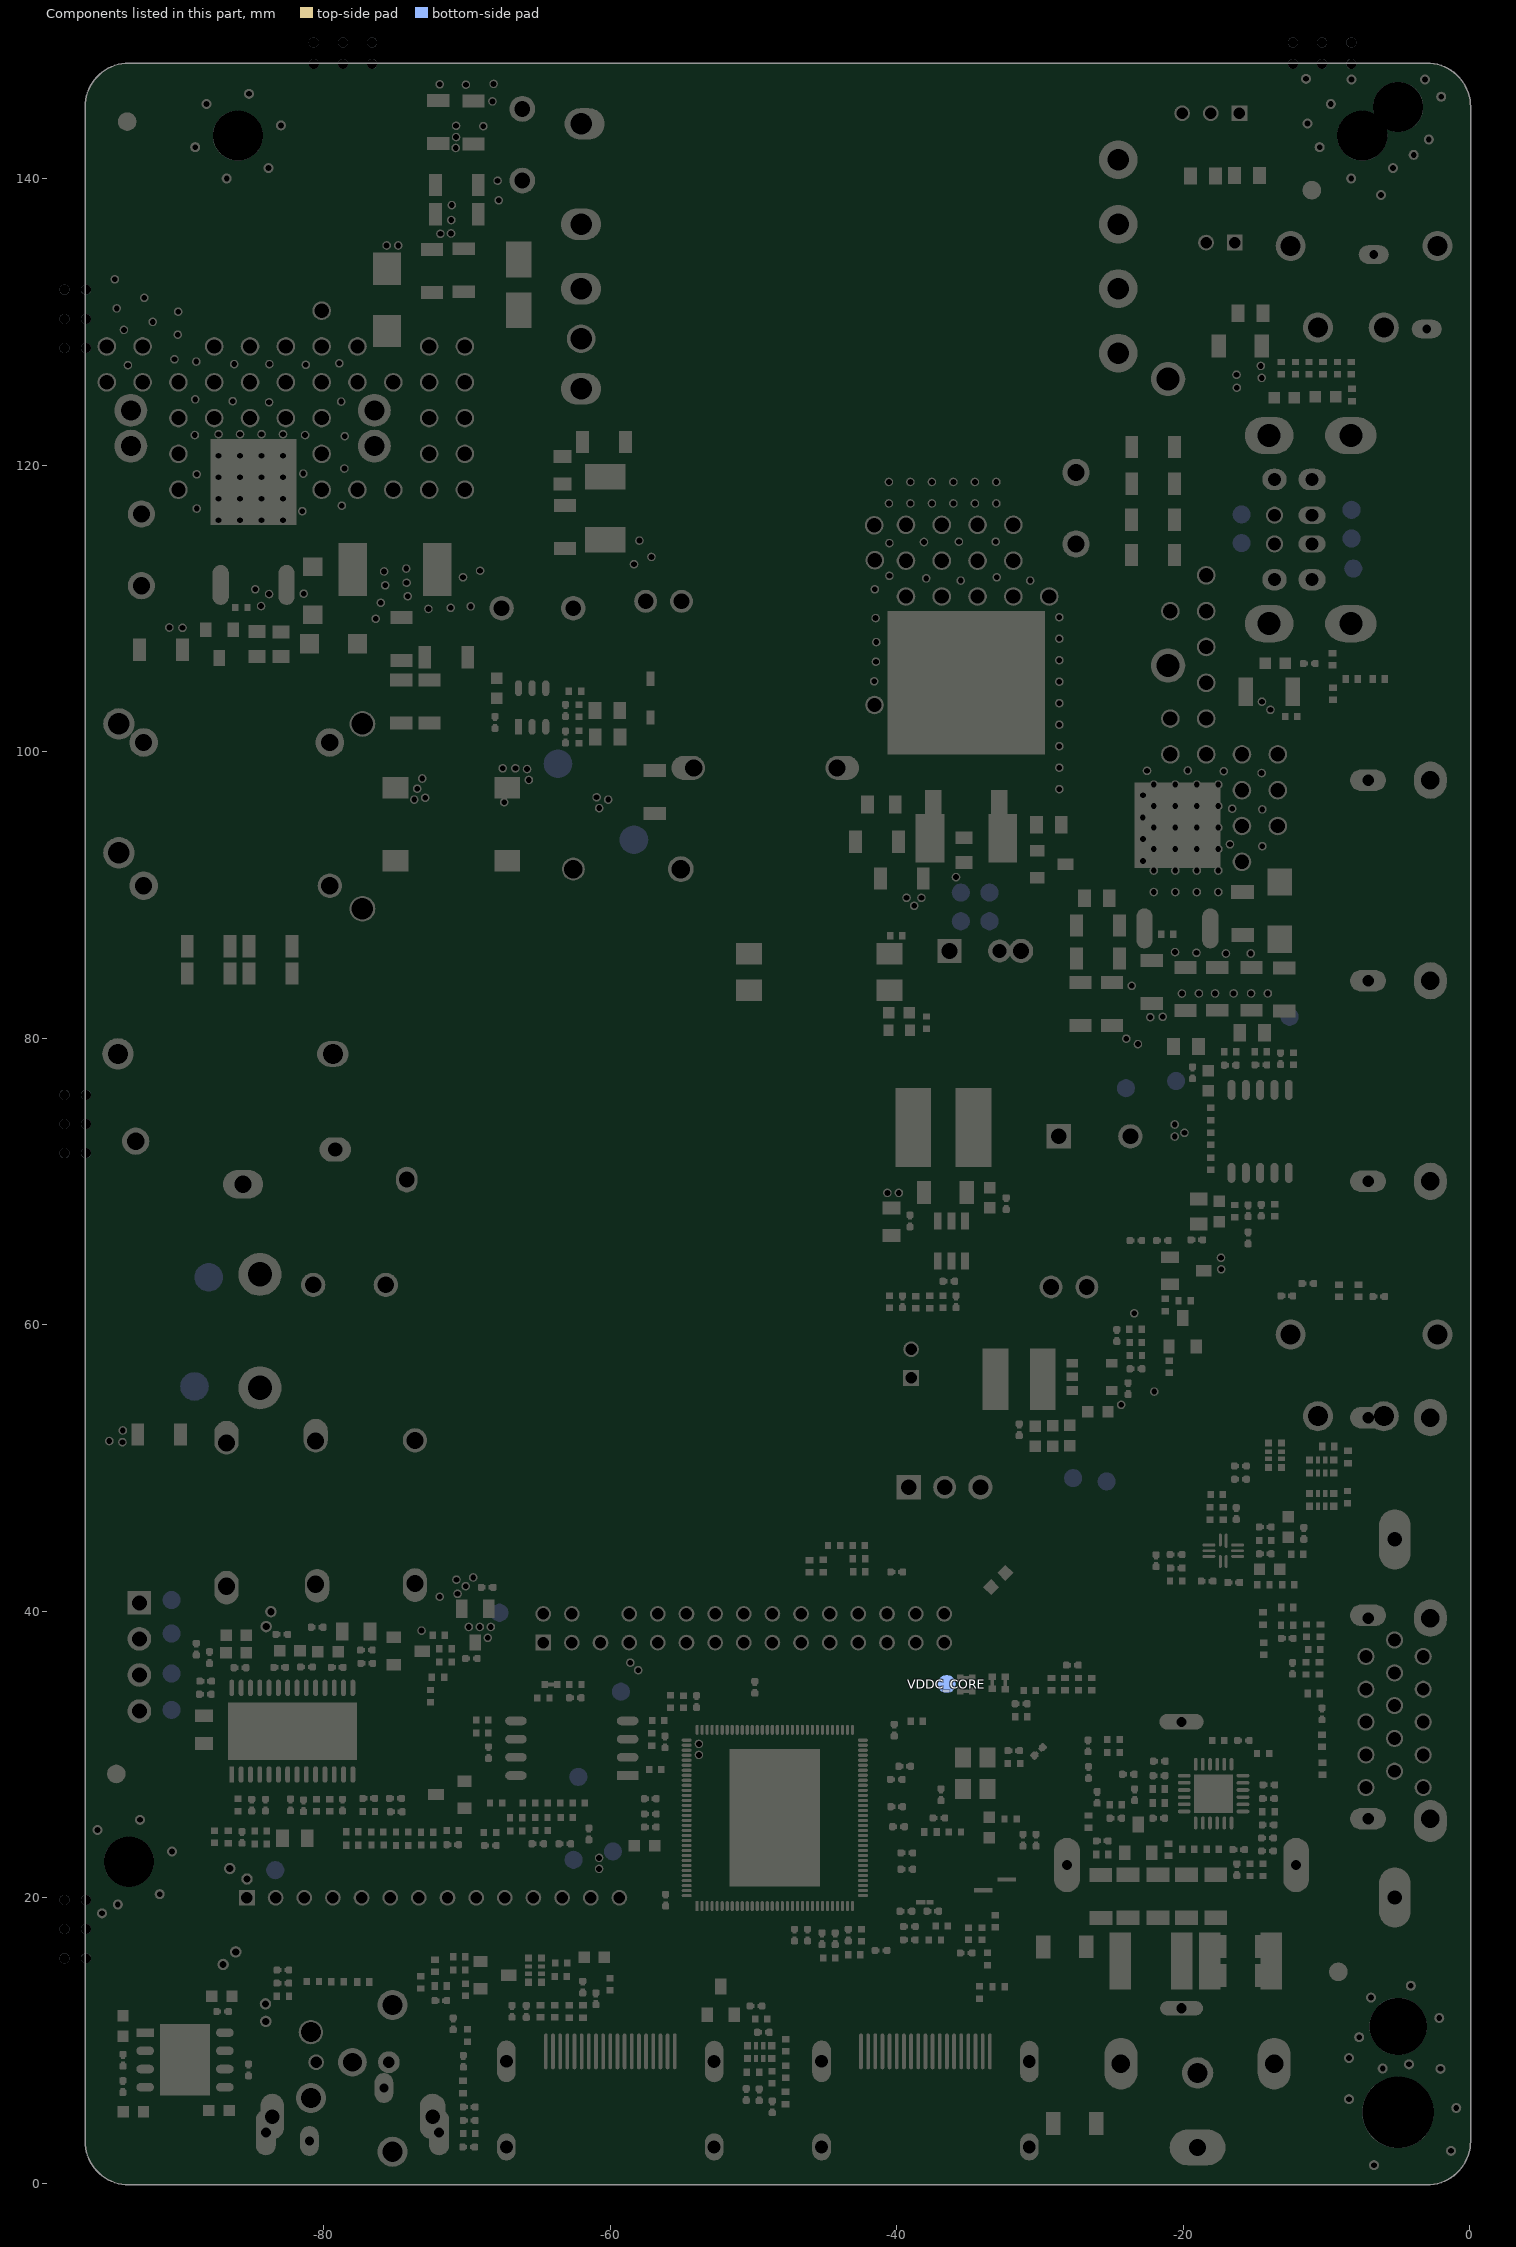
[diagram p0: the components of this part, seen from the top]
# Altium PCB MISC86372.PcbDoc (part 15 of 16)
Units mm, origin at the board's own origin, x right, y up, seen from the top; angles counter-clockwise.
Board outline 96.73 x 148.13 mm, 2 copper layers (TopLayer, BottomLayer), stack 1.571 mm thick; 578 components, 318 nets, 2702 pads, 836 vias.

## Polygon pours and split planes (outlines as drawn)
GND1 on BottomLayer "12mil" (solid, remove dead copper, pour order 1004): -86,138.424 cw(c-86,143) -90.576,143 cw(c-86,143) -86,147.576 cw(c-86,143) -81.424,143 cw(c-86,143)
GND on BottomLayer "gnd" (solid, remove dead copper, pour order 1008): -30.251,70.028 -30.226,70.002 -26.218,70.002 -24.944,68.728 -19.815,68.728 -18.796,67.709 -18.796,66.124 -17.983,65.312 -19.847,63.448 -31.19,63.448 -35.389,67.647
GND on BottomLayer "6.2" (solid, remove dead copper, pour order 1012): -26.924,39.145 -27.254,38.814 -27.254,37.577 -27.334,37.577 -30.556,34.355 -30.556,27.813 -32.173,26.196 -32.173,21.638 -36.246,17.565 -36.246,14.038 -35.281,13.073 -35.281,12.37 -33.859,12.37 -33.2,11.71 -30.354,11.71 -30.048,11.405 -29.896,11.557 -29.896,17.934 -28.753,19.077 -28.753,24.504 -26.684,26.573 -26.684,32.218 -23.749,35.154 -23.749,39.045 -24.023,39.319
RFGND on BottomLayer "fgnd" (solid, remove dead copper, pour order 1006): -26.695,18.924 -26.695,0.279 -25.756,-0.66 -25.019,0.076 -11.963,0.076 -10.566,1.473 -10.566,10.336 -13.514,13.284 -16.459,13.284 -16.713,13.538 -16.713,18.877 -17.14,19.304 -26.316,19.304
GND on BottomLayer "gnd" (solid, remove dead copper, pour order 1007): -12.061,149.04 -13.245,147.856 -13.245,124.669 -15.531,122.383 -15.531,106.123 -12.314,102.906 -12.314,71.785 -18.575,65.525 -23.439,65.525 -32.346,74.432 -32.346,85.184 -34.127,86.965 -38.719,86.965 -40.474,85.21 -40.474,48.456 -45.681,43.249 -67.22,43.249 -68.465,42.004 -95.465,42.004 -97.675,39.794 -97.675,-0.541 -95.236,-2.979 -1.79,-2.979 3.697,2.507 3.697,146.5 1.182,149.014
GND on TopLayer "5" (solid, remove dead copper, pour order 1011): -40.996,67.639 -41.097,67.537 -41.097,63.233 -39.535,61.671 -31.75,61.671 -29.159,64.262 -29.159,69.266 -29.807,69.913 -40.78,69.913 -41.021,69.672
D_QB801 on TopLayer "12mil" (solid, remove dead copper, pour order 1016): -21.971,89.662 -23.495,91.186 -25.984,91.186 -26.264,91.465 -26.264,111.354 -25.705,111.912 -22.962,111.912 -22.403,112.471 -22.403,122.911 -21.717,123.596 -18.161,123.596 -16.891,122.326 -16.891,102.083 -15.748,100.94 -12.852,100.94 -12.192,100.279 -12.192,90.119 -12.649,89.662
GND on TopLayer "6.2" (solid, remove dead copper, pour order 1019): -26.826,38.989 -26.699,38.862 -15.978,38.189 -14.275,36.525 -12.879,35.09 -11.826,35.093 -10.414,35.093 -10.414,35.006 -9.017,33.609 -9.017,30.26 -9.821,29.456 -11.549,29.456 -17.053,34.96 -25.378,34.96 -27.813,37.396 -27.813,39.116
GND on TopLayer "6.2" (solid, remove dead copper, pour order 1018): -10.593,35.069 -10.616,35.093 -12.704,35.093 -13.2,34.597 -12.01,33.407 -12.01,29.648 -9.177,26.815 -8.931,26.815 -8.27,27.476 -8.27,35.296 -8.535,35.56
GND on TopLayer "6.2" (solid, remove dead copper, pour order 1017): -27.338,39.174 -27.674,38.838 -27.674,37.257 -25.52,35.103 -23.524,35.103 -22.966,35.661 -22.966,37.736 -24.24,39.01 -27.138,39.01 -27.352,39.224
VDDC_CORE on TopLayer "12" (solid, remove dead copper, pour order 1003): -58.967,40.919 -59.552,40.335 -59.552,38.684 -59.552,37.363 -58.993,36.805 -59.501,36.297 -59.501,36.22 -60.898,36.22 -61.838,37.16 -61.838,37.77 -61.838,38.684 -60.949,39.573 -60.143,40.379 -60.033,40.379 -59.808,40.605
no net on TopLayer "12mil" (solid, remove dead copper, pour order 1015): -69.494,137.185 -69.494,139.929 -69.113,140.31 -67.793,140.31 -66.624,141.478 -64.926,141.478 -63.361,143.043 -63.361,144.386 -62.763,144.983 -61.446,144.983 -61.062,144.598 -61.062,143.078 -66.649,137.491 -69.165,137.491 -69.291,137.617
GND1 on TopLayer "12mil" (solid, remove dead copper, pour order 1021): -85.968,139.529 cw(c-85.968,143) -89.439,143 cw(c-85.968,143) -85.968,146.471 cw(c-85.968,143) -82.498,143 cw(c-85.968,143)
RFGND on TopLayer "fgnd" (solid, remove dead copper, pour order 1005): -27,19.253 -26.796,19.049 -12.556,19.049 -11.507,18 -11.507,1.726 -12.759,0.474 -25.264,0.474 -27.127,2.337 -27.127,19.098 -27.026,19.2
GND on TopLayer "5" (solid, remove dead copper, pour order 1010): -55.245,20.766 -56.032,19.978 -56.032,16.764 -61.316,11.481 -61.316,10.998 -59.795,10.998 -59.689,10.892 -32.588,10.892 -32.588,11.175 -37.111,15.697 -45.974,15.697 -48.663,18.386 -48.663,20.091
GND on TopLayer "gnd" (solid, remove dead copper, pour order 1009): -12.278,148.971 -12.849,148.4 -12.849,124.943 -13.119,124.943 -15.748,122.314 -15.748,106.054 -11.535,101.841 -11.535,67.615 -13.695,65.456 -24.663,65.456 -32.563,73.355 -32.563,78.411 -40.691,78.411 -40.691,49.428 -46.939,43.18 -67.437,43.18 -68.682,41.935 -95.682,41.935 -97.892,39.726 -97.892,-0.61 -95.453,-3.048 -2.007,-3.048 3.48,2.438 3.48,146.431 0.965,148.946
GND on TopLayer "5" (solid, remove dead copper, pour order 1014): -42.812,31.54 -42.697,31.654 -42.697,33.412 -41.225,34.885 -37.266,34.885 -34.851,37.301 -34.851,40.308 -32.073,43.085 -32.073,44.291 -18.059,58.305 -18.059,61.682 -11.299,68.442 -11.299,104.627 -10.017,105.909 -4.648,108.179 -2.14,106.928 -6.375,102.692 -6.375,102.553 -8.585,100.343 -8.585,66.809 -14.173,61.221 -14.173,56.229 -15.005,55.397 -16.092,55.397 -28.55,42.94 -28.55,41.758 -31.318,38.989 -31.318,33.782 -32.376,32.725 -38.921,32.725 -39.947,31.699 -42.524,31.699

## Keep-outs
KeepOutLayer:
  rectangle: 153.901,36.608 157.208,38.608
  region: -56.845,135.407 -56.845,121.245 ccw(c-54.305,121.245) -56.101,119.449 ccw(c-54.831,120.719) -54.831,118.923 -48.145,118.923 ccw(c-48.145,120.484) -47.041,119.38 ccw(c-47.715,120.055) -46.761,120.055 -46.761,121.107 ccw(c-46.761,121.536) -46.458,121.233 -37.777,129.914 ccw(c-39.573,131.71) -37.033,131.71 -37.033,138.445 ccw(c-39.573,138.445) -37.777,140.241 -38.176,140.64 cw(c-39.648,142.112) -39.648,140.03 -52.299,140.03
  lines w0.127: -101.101,0 -191.7,0 cw(c-191.7,3) -194.7,3 -194.7,145 cw(c-191.7,145) -191.7,148 -101.1,148 cw(c-101.1,145) -98.1,145 -98.1,2.839 ; -101.101,149.5 -191.7,149.5 cw(c-191.7,152.5) -194.7,152.5 -194.7,294.5 cw(c-191.7,294.5) -191.7,297.5 -101.1,297.5 cw(c-101.1,294.5) -98.1,294.5 -98.1,152.339 ; -98.1,70.71 cw(c-97.35,69.96) -96.6,70.71 ; -98.1,77.29 ccw(c-97.35,78.04) -96.6,77.29 ; -98.1,220.21 cw(c-97.35,219.46) -96.6,220.21 ; -98.1,221.25 -98.1,152.5 ; -98.1,226.79 ccw(c-97.35,227.54) -96.6,226.79 ; -96.6,76.25 -96.6,145 cw(c-93.6,145) -93.6,148 -3,148 cw(c-3,145) 0,145 0,3 cw(c-3,3) -3,0 -93.6,0 cw(c-93.6,3) -96.6,3 -96.6,76.338 ; -96.6,219.75 -96.6,152.5 ; -96.6,294.5 cw(c-93.6,294.5) -93.6,297.5 ; -96.6,294.661 -96.6,152.5 ; -93.599,297.5 -3,297.5 ; -86,297.5 -3,297.5 ; 167.894,36.608 167.894,38.608 ; -98.1,152.5 cw(c-101.1,152.5) -101.1,149.5 ccw(c-101.1,152.5) -98.1,152.5 ; -96.6,152.5 ccw(c-93.6,152.5) -93.6,149.5 -3,149.5 ccw(c-3,152.5) 0,152.5 0,294.5 ccw(c-3,294.5) -3,297.5 ; -187.589,148 ccw(c-188.339,148.75) -187.589,149.5 cw(c-188.339,148.75) -187.589,148 ; -181.009,148 cw(c-180.259,148.75) -181.009,149.5 ccw(c-180.259,148.75) -181.009,148 ; -119.232,148 ccw(c-119.982,148.75) -119.232,149.5 cw(c-119.982,148.75) -119.232,148 ; -112.652,148 cw(c-111.902,148.75) -112.652,149.5 ccw(c-111.902,148.75) -112.652,148 ; -101.1,0 ccw(c-101.1,3) -98.1,3 cw(c-101.1,3) -101.1,0 ; -98.1,14.503 cw(c-97.35,13.753) -96.6,14.503 ccw(c-97.35,13.753) -98.1,14.503 ; -98.1,21.083 ccw(c-97.35,21.833) -96.6,21.083 cw(c-97.35,21.833) -98.1,21.083 ; -98.1,126.917 cw(c-97.35,126.167) -96.6,126.917 ccw(c-97.35,126.167) -98.1,126.917 ; -98.1,133.497 ccw(c-97.35,134.247) -96.6,133.497 cw(c-97.35,134.247) -98.1,133.497 ; -98.1,164.003 cw(c-97.35,163.253) -96.6,164.003 ccw(c-97.35,163.253) -98.1,164.003 ; -98.1,170.583 ccw(c-97.35,171.333) -96.6,170.583 cw(c-97.35,171.333) -98.1,170.583 ; -98.1,276.417 cw(c-97.35,275.667) -96.6,276.417 ccw(c-97.35,275.667) -98.1,276.417 ; -98.1,282.997 ccw(c-97.35,283.747) -96.6,282.997 cw(c-97.35,283.747) -98.1,282.997 ; -81.952,148 ccw(c-82.702,148.75) -81.952,149.5 cw(c-82.702,148.75) -81.952,148 ; -75.372,148 cw(c-74.622,148.75) -75.372,149.5 ccw(c-74.622,148.75) -75.372,148 ; -13.595,148 ccw(c-14.345,148.75) -13.595,149.5 cw(c-14.345,148.75) -13.595,148 ; -7.015,148 cw(c-6.265,148.75) -7.015,149.5 ccw(c-6.265,148.75) -7.015,148 ; 153.901,36.608 172.494,36.608 172.494,38.608 153.901,38.608 153.901,36.608
  text "KeepOutLayer" at 157.782,37.14 h1.52
  text ".GKO" at 168.496,37.066 h1.52

## Other copper
TopLayer:
  drawing of 178 lines, arcs and shapes, not listed
  text "TopLayer" at 158.119,52.346 h1.52
  text ".GTL" at 168.52,52.237 h1.52
BottomLayer:
  rectangle net GND: -61.443,36.805 -59.766,39.116
  rectangle net GND: -13.995,18.771 -9.881,24.892
  rectangle net GND: -41.554,37.008 -39.878,42.24
  rectangle net GND: -73.99,1.499 -70.739,7.087
  rectangle net GND: -88.367,40.615 -85.014,42.012
  rectangle: 153.901,46.245 157.208,48.245
  rectangle net GND: -22.271,30.404 -16.358,33.833
  rectangle net GND: -81.712,39.617 -73.228,41.981
  rectangle net GND: -36.79,46.901 -32.388,50.055
  rectangle net GND: -89.586,17.678 -84.15,20.523
  rectangle net GND: -53.569,36.982 -51.867,41.097
  pour cut-out: -18.339,66.294 -18.44,66.294 -18.567,66.167 -18.567,65.913 -17.366,64.711 -17.366,64.665 -17.183,64.665 -16.849,64.999
  region net GND: -6.777,44.195 -6.644,44.327 -6.644,45.141 -6.756,45.253 -6.692,45.318 -5.719,45.318 -5.131,44.729 -5.131,42.062 -5.69,42.062 -6.777,43.149
  region net GND: -3.803,71.119 -2.565,72.356 -2.565,80.823 -4.75,83.007 -4.75,86.335 -3.937,87.147 -3.937,95.885 -4.775,96.723 -4.775,104.394 -6.655,106.274 -15.531,106.274 -15.531,109.513 -14.75,110.294 -10.262,110.294 -9.867,110.689 -6.811,110.689 -6.02,111.481 -6.02,117.551 -5.639,117.932 -6.02,118.313 -14.542,118.313 -15.531,119.303 -15.531,122.383 -13.2,124.714 -8.423,124.714 -6.086,122.377 -6.017,122.377 -1.575,117.935 -1.575,107.594 -0.787,106.807 -0.787,67.666 -2.007,66.446 -3.803,68.243
  region net GND: -69.215,18.923 -69.215,18.085 -68.859,17.729 -68.758,17.831 -67.005,17.831 -67.005,18.009 -66.345,18.669 -66.497,18.821 -66.497,20.498 -66.671,20.671 -67.467,20.671
  pour cut-out: -25.552,0.207 -27.361,0.207 -27.361,13.66 -26.154,14.867 -25.552,14.266 -25.552,7.72
  region net RFGND: -16.189,13.268 -17.12,14.199 -17.678,14.199 -17.678,13.132 -17.932,12.878 -17.45,12.395 -17.094,12.395 -16.205,13.284
  pour cut-out: -15.363,15.514 -13.115,13.267 -13.115,13.056 -15.443,13.056 -15.656,13.268 -16.189,13.268 -16.713,13.792 -16.713,16.162
  pour cut-out: -12.471,9.754 -12.471,-2.413 -12.268,-2.616 -10.663,-1.011 -10.663,10.231 -10.998,10.566 -11.659,10.566
  pour cut-out: -16.305,13.384 -10.663,7.742 -10.663,10.814 -13.321,13.472 -16.217,13.472
  pour cut-out: -26.111,8.992 -26.111,13.36 -23.495,15.977 -16.358,15.977 -15.875,16.459 -15.875,16.967 -16.713,17.805 -24.257,17.805 -27.361,14.701 -27.361,8.133 -26.916,7.688
  region net GND: -33.429,86.981 -33.859,86.551 -33.859,83.347 -32.688,82.175 -31.817,82.175 -31.182,82.809 -31.182,86.046
  pour cut-out: -16.236,17.328 -14.859,15.951 -14.859,14.3 -15.824,14.3 -18.562,17.038
  pour cut-out: -17.094,118.313 -7.468,118.313 -6.477,117.323 -6.477,111.531 -7.319,110.689 -16.467,110.689 -16.996,110.16 -17.526,110.689 -17.526,119.228 -17.297,119.456 -15.685,119.456 -14.491,118.262 -17.043,118.262
  region net MINIAV_LOUT&OPT: -76.124,8.6 -76.124,7.366 -76.251,7.239 -75.712,6.7 -75.139,6.7 -74.701,7.137 -74.701,8.636 -74.955,8.89 -75.971,8.89
  region net AVOUT: -82.089,11.328 -81.988,11.43 -79.816,11.43 -79.702,11.316 -79.702,9.931 -79.854,9.779 -81.949,9.779 -82.089,9.919
  region net SPDIF_OUT: -79.943,8.966 -81.568,8.966 -81.695,8.839 -81.695,8.103 -81.568,7.976 -79.917,7.976 -79.816,8.077 -79.816,8.839
  region net 12V: -42.107,52.829 -42.85,52.086 -42.85,47.724 -41.027,47.724 -39.859,48.892 -40.489,49.522 -40.489,52.981
  region net 12V: -41.224,70.891 -41.224,70.485 -40.767,70.028 -39.776,70.028 -39.472,69.723 -39.472,68.669 -39.713,68.428 -40.589,68.428 -41.097,67.92 -41.631,68.453 -41.631,70.891
  region net GND: 213 vertices and 0 holes, not listed, extent -87.242,19.472 -85.365,20.508
  region net GND: -27.889,20.269 -27.737,20.422 -27.737,24.536 -27.017,24.536 -25.984,23.504 -25.984,21.361 -27.33,20.015 -28.105,20.015
  pour cut-out: -17.573,64.52 -14.286,64.888 -14.286,66.021 -13.564,66.743 -13.564,68.529 -17.048,68.529 -18.339,67.238 -18.339,66.294
  region net 12V: -34.874,86.919 -34.874,91.389 -39.441,95.956 -39.441,99.36 -42.52,102.438 -42.52,118.262 -33.376,127.406 -33.376,133.121 -31.014,135.483 -23.869,135.483 -23.19,136.161 -23.19,137.433 -23.924,138.166 -31.988,138.166 -35.712,134.442 -35.712,128.93 -44.78,119.863 -44.78,101.778 -42.088,99.085 -42.088,95.352 -37.719,90.983 -37.719,87.173 -38.176,86.716 -37.541,86.081 -35.712,86.081
  region net L-3: -81.178,68.783 -86.589,68.783 -87.02,69.215 -87.02,76.962 -84.176,79.807 -78.867,79.807 -78.41,79.35 -78.41,77.876 -79.121,77.165 -82.144,77.165 -83.896,75.413 -83.896,71.704 -83.287,71.704 -81.128,73.863 -78.359,73.863 -77.546,73.05 -77.546,72.415
  region net GND: -89.377,42.697 -72.949,42.697 -72.565,42.313 -72.565,40.643 -72.822,40.386 -74.136,40.386 -75.126,41.377 -77.902,41.377 -79.476,39.802 -81.49,39.802 -82.882,41.195 -85.475,41.195 -86.157,40.513 -87.573,40.513 -89.555,42.494 -90.241,42.494
  region net L: -81.497,95.693 -80.915,93.991 -80.364,95.693
  region net L: -83.722,95.693 -83.14,93.991 -82.589,95.693
  region net L: -82.605,95.693 -82.022,93.991 -81.471,95.693
  region net L-3: -80.342,91.389 -80.924,93.091 -81.475,91.389
  region net L-3: -81.45,91.389 -82.032,93.091 -82.583,91.389
  region net L-3: -82.558,91.389 -83.14,93.091 -83.691,91.389
  region net L: -77.216,103.022 -81.102,103.022 -83.744,100.381 -83.744,95.656 -83.515,95.428 -80.645,95.428 -80.391,95.682 -80.391,98.298 -77.927,100.762 -76.962,100.762 -76.327,101.397 -76.327,102.489 -76.835,102.997 -76.937,102.997
  region net L-3: -80.467,88.062 -83.691,91.286 -83.691,91.62 -83.363,91.948 -78.867,91.948 -76.352,89.433 -76.352,88.468 -76.759,88.062
  region net L-2: -76.429,62.586 -76.429,69.444 -74.905,70.968 -74.016,70.968 -73.711,70.663 -73.711,61.087 -73.99,60.808 -75.057,60.808 -76.403,62.154 -76.403,62.611
  region net L-1: -87.427,65.329 -82.169,65.329 -79.959,63.119 -79.959,62.306 -80.797,61.468 -87.935,61.468 -89.027,62.56 -89.027,64.694 -88.367,65.354 -87.452,65.354
  region net GND: -30.936,87.071 -29.273,85.408 -29.273,83.884 -30.81,82.347 -30.81,77.902 -27.61,74.701 -27.61,72.542 -27.838,72.314 -29.515,72.314 -32.062,74.861 -32.062,77.173 -32.062,83.878 -33.579,85.395 -33.579,86.563 -33.071,87.071
  region net GND: -19.99,80.391 -20.938,81.339 -22.649,81.339 -21.209,79.899 -21.209,73 -20.838,72.628 -20.234,72.628 -19.99,72.873
  region net GND: -44.882,99.568 -44.882,94.463 -40.97,90.551 -40.97,88.57 -40.437,88.036 -38.76,88.036 -38.069,88.728 -38.069,90.693 -42.545,95.169 -42.545,99.111 -43.307,99.873 -44.602,99.873 -44.856,99.619
  region net GND: -34.214,90.653 -34.214,86.995 -33.579,86.36 -33.579,85.649 -31.09,85.649 -30.124,84.684 -30.124,86.36 -32.257,88.492 -32.257,90.524 -32.766,91.034 -33.858,91.034 -34.239,90.653
  region net N-1: -83.617,53.289 -85.903,53.289 -86.741,54.127 -90.473,54.127 -93.165,51.435 -94.894,51.435 -95.377,51.918 -95.377,52.787 -94.666,53.498 -94.666,65.989 -95.733,67.056 -95.733,93.243 -95.072,93.904 -92.329,93.904 -91.262,92.837 -91.262,80.34 -92.431,79.172 -93.167,79.172 -93.193,79.146 -93.193,78.765 -92.481,78.765 -91.669,77.953 -91.669,69.139 -92.481,68.326 -92.481,60.173 -89.941,57.633 -83.591,57.633 -82.499,56.54 -82.499,54.407
  region net NetCB102_1: -59.69,111.531 -59.69,115.722 -59.461,115.951 -58.569,115.951 -56.281,113.663 -56.281,111.689 -56.845,111.125 -56.845,110.16 -57.277,109.728 -57.887,109.728
  region net GND: -24.536,84.938 -24.536,83.261 -21.26,79.985 -20.853,79.985 -20.853,81.255 -23.104,83.505
  region net GND: -20.717,72.679 -20.133,72.679 -19.609,73.203 -19.609,73.889 -20.409,74.689 -20.714,74.689
  region net FB: -20.625,81.991 -20.625,83.515 -20.295,83.845 -14.402,83.845 -13.759,84.488 -13.754,85.492 -14.571,86.309 -22.835,86.309 -23.231,85.913 -23.231,84.598
  region net GND: -13.382,80.112 -18.796,80.112 -20.422,81.737 -20.422,83.16 -20.142,83.439 -13.691,83.439 -13.382,83.131
  region net GND: -13.964,81.587 -12.802,80.425 -12.802,75.438 -14.3,73.939 -14.3,67.818 -16.332,65.786 -17.526,65.786 -18.051,66.311 -18.051,68.589 -16.88,69.759 -16.88,71.522 -18.263,72.904 -18.263,79.391 -18.038,79.616 -14.719,79.616 -14.389,79.946 -14.389,81.587
  region net NetCNB821_2: 213 vertices and 0 holes, not listed, extent -21.958,144.043 -20.081,145.08
  region net N-1: -94.678,90.957 -95.834,92.114 -95.834,94.005 -95.707,94.132 -91.524,94.132 -91.262,93.871 -91.262,91.669 -92.1,90.83 -92.253,90.983 -94.615,90.983
  region net N-1: -93.56,93.943 -94.142,95.645 -94.693,93.943
  region net N-1: -91.335,93.943 -91.917,95.645 -92.468,93.943
  region net N-1: -92.452,93.943 -93.034,95.645 -93.585,93.943
  region net N-1: -94.668,93.943 -95.25,95.645 -95.801,93.943
  pour cut-out: -79.759,11.373 -77.581,9.195 -75.8,9.195 -75.8,7.034 -75.659,6.893 -75.659,5.994 -77.241,5.994 -79.959,3.277 -80.823,4.14 -80.823,10.777 -81.095,11.049
  region net 12V: -67.539,44.069 -69.444,44.069 -71.12,42.393 -71.12,41.173 -70.866,40.919 -70.358,40.919 -68.91,42.367 -67.488,42.367 -67.488,44.018
  region net 12V: -69.525,41.95 -68.091,41.95 -67.568,42.473 -68.665,43.57 -69.291,43.57 -69.291,43.459 -69.901,42.85 -69.901,42.291
  region net 5V_M: -15.621,64.11 -16.18,63.551 -17.501,63.551 -17.678,63.729 -17.678,64.795 -17.475,64.999 -16.224,64.999 -15.919,64.694 -15.596,64.694 -15.596,64.668 -15.57,64.643
  region net D_QB801: -12.62,86.999 -12.23,87.389 -12.23,99.369 -17.094,104.233 -17.094,117.881 -17.805,118.593 -19.05,118.593 -20.777,116.865 -20.777,111.684 -23.114,109.347 -23.114,88.214 -21.899,86.999
  region net D_QB101: -79.451,115.621 -80.264,114.808 -95.481,114.808 -95.91,115.237 -95.91,134.3 -95.626,134.584 -95.428,134.584 -94.645,133.81 -94.209,133.304 -93.701,132.918 -93.155,132.583 -92.877,132.359 -92.38,132.105 -91.732,131.775 -91.288,131.504 -90.043,131.011 -89.56,130.835 -89.031,130.67 -88.495,130.556 -87.791,130.429 -87.225,130.353 -85.703,130.353 -84.887,130.404 -84.303,130.46 -83.75,130.581 -82.935,130.759 -82.321,130.937 -81.772,131.115 -81.001,131.369 -80.416,131.661 -70.315,131.661 -69.278,130.624 -69.278,130.556 -69.266,130.543 -69.266,121.285 -66.65,118.669 -66.65,116.732 -67.761,115.621
  region net NetCB114_2: -65.608,144.729 -71.145,144.729 -72.669,146.253 -72.669,147.168 -72.392,147.445 -65.962,147.445 -65.031,146.514 -65.031,145.306
  region net SNB-D: -75.59,134.544 -75.937,134.624 -76.073,135.306 -75.641,135.941 -75.057,136.83 -74.549,137.846 -74.219,138.582 -73.431,139.141 -72.644,139.852 -71.984,140.894 -71.704,141.707 -71.577,143.307 -71.66,144.221 -68.595,144.221 -68.351,143.978 -68.351,142.85 -73.406,137.795 -73.406,135.484 -74.346,134.544
  region net Vbridge: -61.036,97.13 -59.995,97.13 -55.076,92.211 -55.076,90.865 -55.042,90.83 -58.471,90.83 -58.928,91.288 -58.928,93.777 -60.884,95.733 -61.239,96.088 -61.239,96.926
  region net Vbridge: -66.878,134.163 -66.878,135.509 -68.199,136.83 -68.199,139.954 -66.573,141.58 -64.824,141.58 -63.246,143.158 -63.246,144.323 -62.586,144.983 -61.138,144.983 -60.554,144.399 -60.554,143.565 -65.684,138.434 -65.684,135.052 -66.167,134.569
  region net SNB-RM: -69.774,134.62 -69.774,139.192 -69.875,139.294 -70.409,139.294 -72.136,137.566 -72.136,134.315 -71.907,134.087 -70.282,134.087 -69.799,134.569
  region net SGND: -67.843,107.544 -64.465,104.165 -64.465,103.429 -66.529,103.429 -67.52,104.419 -67.469,104.47 -67.469,106.356 -67.97,106.858 -79.477,106.858 -79.985,107.366 -79.985,109.88 -79.502,110.363 -79.339,110.2 -78.471,110.2 -79.4,109.271 -79.4,108.282 -78.662,107.544
  region net SGND: -67.907,99.902 -65.098,99.902 -63.519,101.481 -63.519,102.864 -65.739,105.084 -66.406,105.084 -67.11,105.788 -68.47,104.429 -68.47,102.607 -67.259,101.397 -67.259,100.55
  region net SGND: -67.767,98.984 -67.767,95.58 -63.779,91.592 -63.779,91.059 -63.221,90.5 -61.722,90.5 -61.316,90.907 -61.316,92.304 -62.027,93.015 -63.398,93.015 -65.1,94.717 -65.1,99.187 -65.557,99.644 -67.107,99.644
  region net SGND: -77.318,109.068 -76.937,108.687 -66.599,108.687 -66.319,108.966 -66.319,111.328 -68.072,113.081 -77.546,113.081 -79.883,110.744 -79.883,109.144 -79.629,109.398 -77.597,109.398 -77.292,109.093
  region net N-2: -95.832,98.248 -95.25,96.545 -94.699,98.248
  region net N-2: -92.499,98.248 -91.917,96.545 -91.366,98.248
  region net N-2: -93.607,98.248 -93.025,96.545 -92.474,98.248
  region net N-2: -94.715,98.248 -94.132,96.545 -93.581,98.248
  region net N-2: -95.86,102.311 -95.86,98.247 -95.707,98.095 -90.5,98.095 -88.849,96.444 -88.849,90.856 -87.147,90.856 -86.817,91.186 -86.817,97.409 -92.38,102.972 -95.171,102.972 -95.857,102.286
  region net N-2: -76.632,84.76 -75.366,84.76 -73,87.126 -73,90.68 -77.216,94.896 -77.216,97.104 -76.708,97.612 -75.743,97.612 -74.6,98.755 -73.152,98.755 -72.542,98.146 -72.542,92.939 -71.069,91.465 -71.069,80.442 -71.476,80.035 -72.415,80.035 -75.722,83.342 -77.694,83.342 -77.694,83.926 -77.318,84.303
  region net NetDB109_A: -82.677,111.735 -89.306,111.735 -91.135,109.906 -91.135,108.56 -90.881,108.306 -89.814,108.306 -88.341,109.779 -81.625,109.779 -81.026,110.378 -81.026,111.118 -81.643,111.735
  region net GND: -29.117,23.332 -29.117,20.57 -27.572,19.025 -26.181,20.416 -25.044,20.416 -25.044,22.708 -24.663,23.089 -26.238,24.663 -27.786,24.663
  region net LED_FB: 213 vertices and 0 holes, not listed, extent -20.285,135.016 -18.408,136.053
  region net SYN: -28.342,92.409 -29.566,91.186 -31.801,91.186 -32.664,92.05 -34.849,92.05 -39.014,96.215 -39.014,99.339 -42.189,102.514 -42.189,117.805 -29.413,130.581 -29.413,125.578 -29.413,114.875 -30.277,114.011 -30.277,112.664 -28.342,110.729
  region net SYN: -28.746,133.68 -32.788,129.638 -32.788,125.933 -31.496,125.933 -26.949,130.48 -24.435,130.48 -23.198,131.717 -23.198,132.899 -23.979,133.68
  region net VDDC_CORE: -53.67,29.642 -53.518,29.794 -53.518,30.867 -53.664,31.013 -53.98,31.013 -54.107,30.886 -55.169,30.886 -55.397,31.115 -55.418,31.094 -55.91,31.094 -55.91,30.561 -55.474,30.124 -54.407,30.124 -53.924,29.642
  region net VCC_PANEL: -66.527,37.08 -68.517,37.08 -70.517,38.28 -70.517,39.38 -68.517,40.58 -66.527,40.58
  region net GND: -82.424,3.341 -82.728,3.645 -82.728,6.313 -82.686,6.355 -83.417,7.087 -85.954,7.087 -86.868,6.172 -86.131,5.436 -86.131,1.575 -85.268,0.711 -83.464,0.711 -82.424,1.751
  region net VDDC_CORE: -58.278,36.703 -58.729,36.703 -58.903,36.529 -58.903,36.245 -58.528,35.871 -58.054,35.871 -58.039,35.886 -58.039,36.432
  text ".GBL" at 168.511,46.796 h1.52
  text "BottomLayer" at 157.782,46.758 h1.52